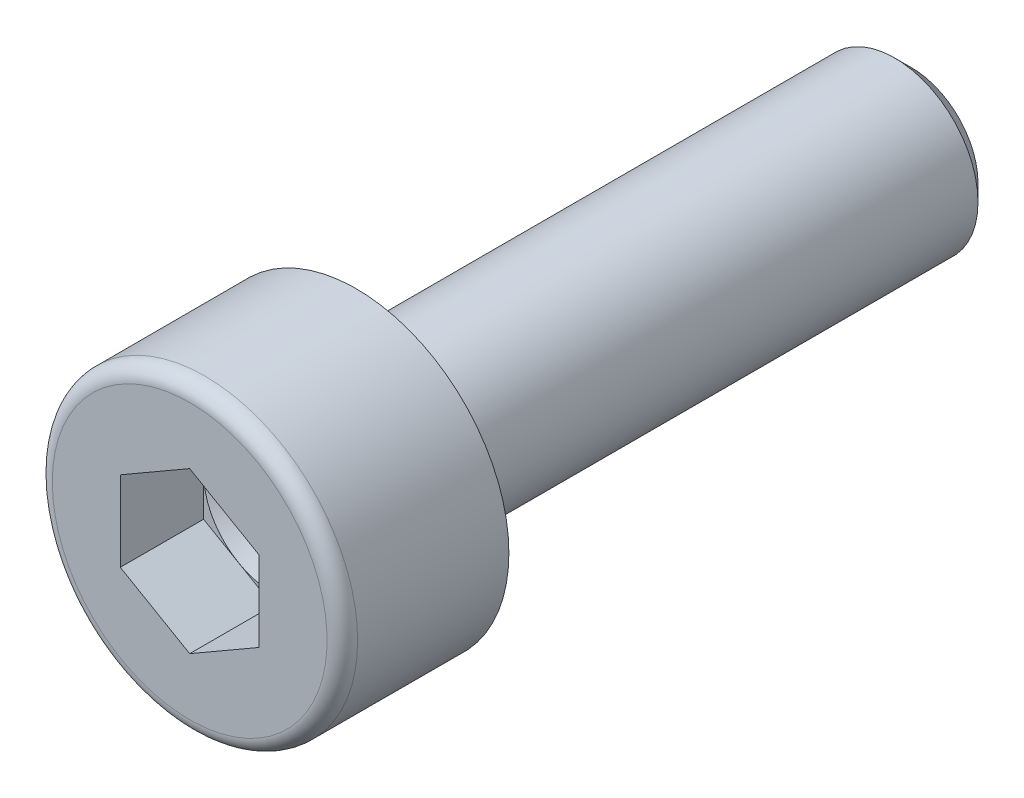
SolidWorks part; units mm, degrees
ref_plane "Front Plane" through (0, 0, 0) normal (0, 0, 1) x (1, 0, 0)
ref_plane "Top Plane" through (0, 0, 0) normal (0, 1, 0) x (1, 0, 0)
ref_plane "Right Plane" through (0, 0, 0) normal (1, 0, 0) x (0, 0, -1)
sketch "Sketch1" plane through (0, 0, 0) normal (1, 0, 0) x (0, 0, -1)
  line L0 (-3, 0) -> (10, 0) construction
  line L1 (-3, 0) -> (-3, 2.75)
  line L2 (-3, 2.75) -> (0, 2.75)
  line L3 (0, 2.75) -> (0, 1.5)
  line L4 (0, 1.5) -> (10, 1.5)
  line L5 (10, 1.5) -> (10, 0)
  point P3 (0, 1.5)
  point P8 (-1.5, 0)
  point P9 (0.125, 1.5)
  point P10 (10, 0.6)
  dimension "A" = 5.5
  dimension "E" = 3
  dimension "L" = 10
  dimension "M" = 3
  dimension "t" = 1.5
  dimension "r" = 0.125
  dimension "(d)" = 1.2
sketch "Sketch2" plane through (0, 0, 0) normal (0, 0, 1) x (1, 0, 0)
  line L1 (0, 1.4434) -> (-1.25, 0.7217)
  line L2 (-1.25, 0.7217) -> (-1.25, -0.7217)
  line L3 (-1.25, -0.7217) -> (0, -1.4434)
  line L4 (0, -1.4434) -> (1.25, -0.7217)
  line L5 (1.25, -0.7217) -> (1.25, 0.7217)
  line L6 (1.25, 0.7217) -> (0, 1.4434)
  circle A0 centre (0, 0) radius 1.25 construction
  dimension "B" = 2.5
sketch "Sketch3" plane through (0, 0, 0) normal (1, 0, 0) x (0, 0, -1)
  line L0 (-3, 0) -> (-3, 2.75) construction
  line L1 (-3, 2.75) -> (0, 2.75) construction
  line L2 (0, 1.5) -> (10, 1.5) construction
  line L3 (0, 2.75) -> (0, 1.5) construction
  line L5 (10, 1.5) -> (10, 0) construction
  line L6 (-3, 0.6) -> (-3, 2.75)
  line L7 (-3, 2.75) -> (0, 2.75)
  line L8 (0, 1.5) -> (10, 1.5)
  line L9 (0, 2.75) -> (0, 1.5)
  line L10 (10, 0.6) -> (-3, 0.6)
  line L11 (10, 1.5) -> (10, 0.6)
revolve "Revolve1" add sketch "Sketch3" angle 360 about L0
cosmetic thread "Cosmetic-Thread1" parameters "D1"=9.875, "D2"=2.55
sketch "Sketch4" plane through (0, 0, 3) normal (0, 0, 1) x (1, 0, 0)
  line L0 (0, 1.4434) -> (-1.25, 0.7217) construction
  line L1 (-1.25, 0.7217) -> (-1.25, -0.7217) construction
  line L2 (-1.25, -0.7217) -> (0, -1.4434) construction
  line L3 (0, -1.4434) -> (1.25, -0.7217) construction
  line L4 (1.25, -0.7217) -> (1.25, 0.7217) construction
  line L5 (1.25, 0.7217) -> (0, 1.4434) construction
  line L6 (0, 1.4434) -> (-1.25, 0.7217)
  line L7 (-1.25, 0.7217) -> (-1.25, -0.7217)
  line L8 (-1.25, -0.7217) -> (0, -1.4434)
  line L9 (0, -1.4434) -> (1.25, -0.7217)
  line L10 (1.25, -0.7217) -> (1.25, 0.7217)
  line L11 (1.25, 0.7217) -> (0, 1.4434)
extrude "Cut-Extrude1" cut sketch "Sketch4" against normal blind 1.5
fillet "Fillet1" radius 0.275 1 edges at (2.75, 0, 3)
chamfer "Chamfer1" distance 0.3 angle 45 1 edges at (1.5, 0, -10)
sketch "Sketch5" plane through (0, 0, 1.5) normal (0, 0, 1) x (1, 0, 0)
  line L6 (1.25, 0.7217) -> (0, 1.4434)
  line L7 (0, 1.4434) -> (-1.25, 0.7217)
  line L8 (-1.25, 0.7217) -> (-1.25, -0.7217)
  line L9 (-1.25, -0.7217) -> (0, -1.4434)
  line L10 (0, -1.4434) -> (1.25, -0.7217)
  line L11 (1.25, -0.7217) -> (1.25, 0.7217)
  line L12 (1.25, 0.7217) -> (0, 1.4434) construction
  line L13 (0, 1.4434) -> (-1.25, 0.7217) construction
  line L14 (-1.25, 0.7217) -> (-1.25, -0.7217) construction
  line L15 (-1.25, -0.7217) -> (0, -1.4434) construction
  line L16 (0, -1.4434) -> (1.25, -0.7217) construction
  line L17 (1.25, -0.7217) -> (1.25, 0.7217) construction
  circle A0 centre (0, 0) radius 1.25
  dimension "D1" = 0
extrude "Cut-Extrude2" cut sketch "Sketch5" against normal blind 10 draft 60
fillet "Fillet2" radius 0.125 1 edges at (1.5, 0, 0)
